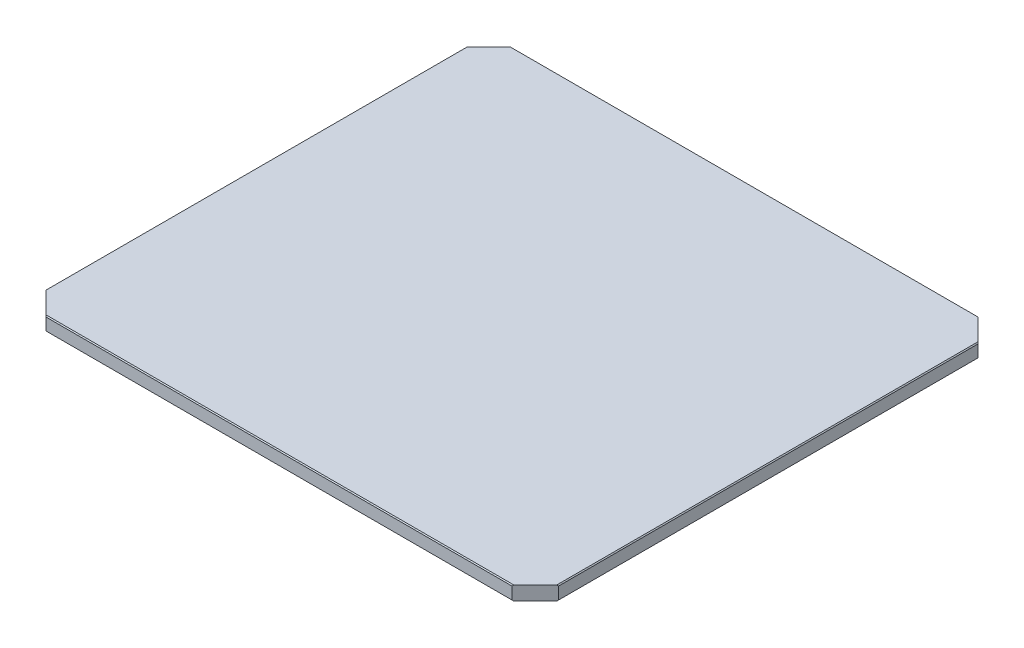
from build123d import *

# Parameters (mm, degrees)
SKETCH1_W      = 110
SKETCH1_H      = 100
EXTRUDE1_DEPTH = 3
CHAMFER1_SIZE  = 5
CHAMFER2_SIZE  = 0.2


with BuildPart() as part:
    # Sketch1 → Extrude1 (new body)
    with BuildSketch(Plane(origin=(0, 0, 0), x_dir=(1, 0, 0), z_dir=(0, 1, 0))):
        Rectangle(SKETCH1_W, SKETCH1_H)
    extrude(amount=EXTRUDE1_DEPTH)

    # Chamfer1
    chamfer1_edges = [part.edges().sort_by_distance(p)[0] for p in [
        (-55, 1.5, -50),
        (55, 1.5, -50),
        (55, 1.5, 50),
        (-55, 1.5, 50),
    ]]
    chamfer(chamfer1_edges, length=CHAMFER1_SIZE)

    # Chamfer2
    chamfer2_edges = [part.edges().sort_by_distance(p)[0] for p in [
        (0, 0, 50),
        (0, 3, 50),
        (-55, 0, 0),
        (0, 0, -50),
        (55, 0, 0),
        (-55, 3, 0),
        (55, 3, 0),
        (0, 3, -50),
    ]]
    chamfer(chamfer2_edges, length=CHAMFER2_SIZE)


solid = part.part
